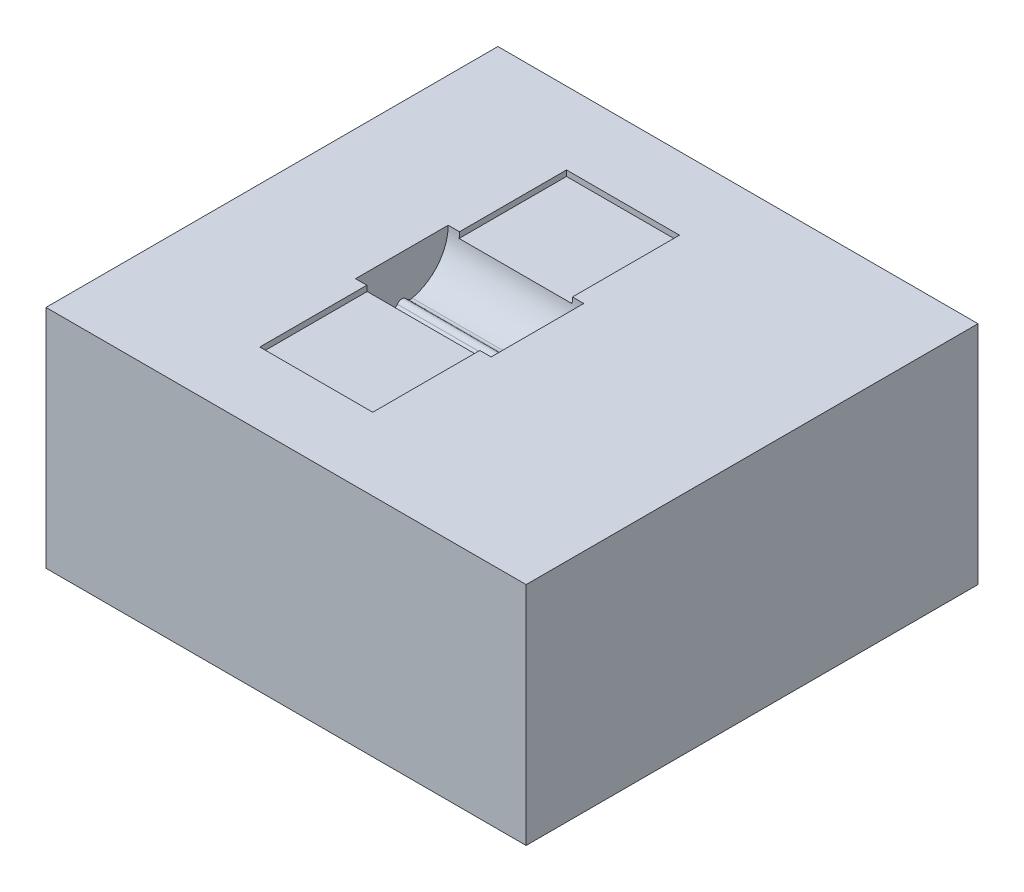
from build123d import *

# Parameters (mm, degrees)
SKETCH1_W                   = 85
SKETCH1_H                   = 80
BOSS_EXTRUDE1_DEPTH         = 40
M8_TAPPED_HOLE1_D           = 6.8
M8_TAPPED_HOLE1_DEPTH       = 22.25
M8_TAPPED_HOLE1_CSINK_D     = 8.05
M8_TAPPED_HOLE1_CSINK_ANGLE = 90
M8_TAPPED_HOLE1_TIP         = 2.042926105
SKETCH5_W                   = 20
SKETCH5_H                   = 54.3
CUT_EXTRUDE1_DEPTH          = 1
CUT_EXTRUDE2_DEPTH          = 12


with BuildPart() as part:
    # Sketch1 → Boss-Extrude1 (new body)
    with BuildSketch(Plane(origin=(0, 0, 0), x_dir=(1, 0, 0), z_dir=(0, 1, 0))):
        Rectangle(SKETCH1_W, SKETCH1_H)
    extrude(amount=BOSS_EXTRUDE1_DEPTH)

    # M8 Tapped Hole1
    with Locations(Plane(origin=(0, 0, 0), x_dir=(-1, 0, 0), z_dir=(0, -1, 0))):
        with Locations((7.5, 28), (-22.5, 0), (7.5, -28), (32.5, 0)):
            CounterSinkHole(M8_TAPPED_HOLE1_D / 2, M8_TAPPED_HOLE1_CSINK_D / 2, depth=M8_TAPPED_HOLE1_DEPTH, counter_sink_angle=M8_TAPPED_HOLE1_CSINK_ANGLE)
            with Locations((0, 0, -(M8_TAPPED_HOLE1_DEPTH + M8_TAPPED_HOLE1_TIP / 2))):  # 118° drill point
                Cone(0, M8_TAPPED_HOLE1_D / 2, M8_TAPPED_HOLE1_TIP, mode=Mode.SUBTRACT)

    # Sketch5 → Cut-Extrude1 (cut)
    with BuildSketch(Plane(origin=(0, 40, 0), x_dir=(1, 0, 0), z_dir=(0, 1, 0))):
        with Locations((-7.5, 0)):
            Rectangle(SKETCH5_W, SKETCH5_H)
    extrude(amount=-CUT_EXTRUDE1_DEPTH, mode=Mode.SUBTRACT)

    # Sketch6 → Cut-Extrude2 (cut, symmetric)
    with BuildSketch(Plane.ZY.offset(7.5)):
        with BuildLine():
            Line((-8.2, 40), (8.2, 40))
            ThreePointArc((8.2, 40), (6.414845549, 34.892186713), (1.836644737, 32.008333333))
            ThreePointArc((1.836644737, 32.008333333), (1.264123473, 32.045632996), (0.806331836, 32.391463415))
            ThreePointArc((0.806331836, 32.391463415), (0, 32.8), (-0.806331836, 32.391463415))
            ThreePointArc((-0.806331836, 32.391463415), (-1.264123473, 32.045632996), (-1.836644737, 32.008333333))
            ThreePointArc((-1.836644737, 32.008333333), (-6.414845549, 34.892186713), (-8.2, 40))
        make_face()
    extrude(amount=CUT_EXTRUDE2_DEPTH, both=True, mode=Mode.SUBTRACT)


solid = part.part
